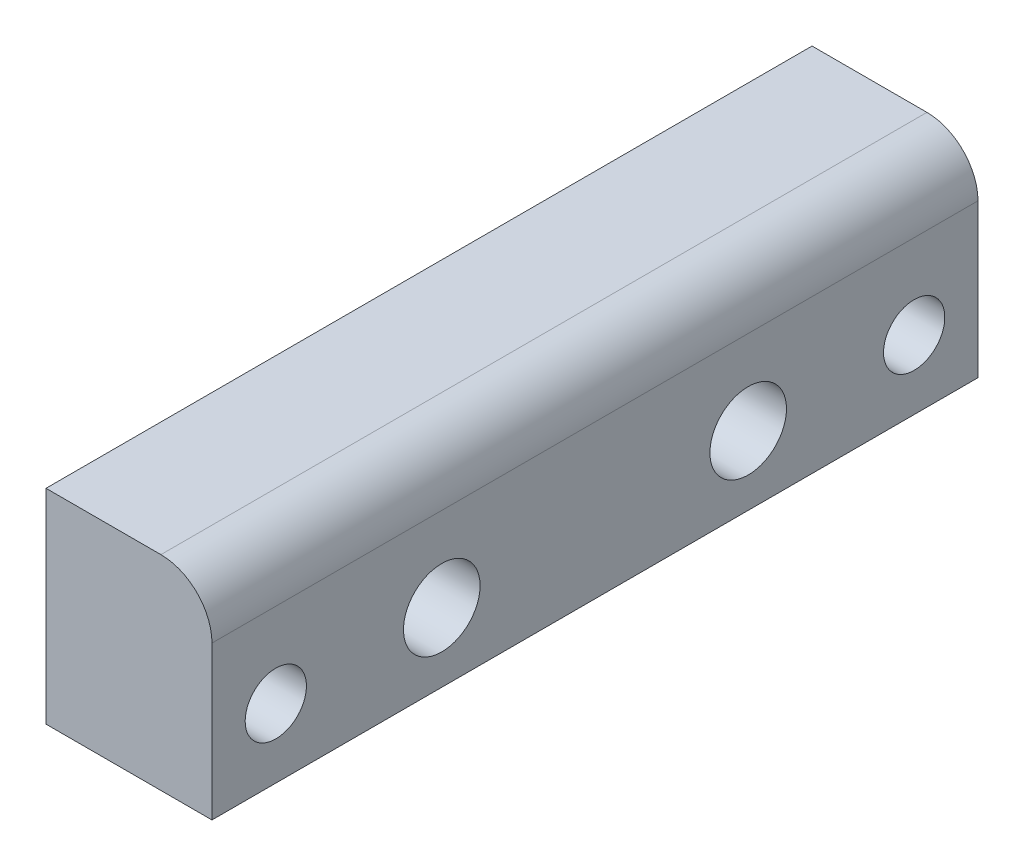
SolidWorks part; units mm, degrees
ref_plane "前视基准面" through (0, 0, 0) normal (0, 0, 1) x (1, 0, 0)
ref_plane "上视基准面" through (0, 0, 0) normal (0, 1, 0) x (1, 0, 0)
ref_plane "右视基准面" through (0, 0, 0) normal (1, 0, 0) x (0, 0, -1)
ref_plane "基准面1" through (3.25, 0, 0) normal (1, 0, 0) x (0, 0, -1)
sketch "草图1" plane through (3.25, 0, 0) normal (1, 0, 0) x (0, 0, -1)
  line L0 (0, -4) -> (0, 4)
  line L1 (0, 4) -> (-30, 4)
  line L2 (-30, 4) -> (-30, -4)
  line L3 (-30, -4) -> (0, -4)
  dimension "D1" = 30
  dimension "D2" = 8
extrude "凸台-拉伸1" add sketch "草图1" against normal blind 6.5
hole_wizard "Ø3.0 (3) 直径孔1" positions "草图3" profile "草图2" hole size "Ø3.0" standard "ANSI Metric"
sketch "草图3" plane through (3.25, 0, 0) normal (1, 0, 0) x (0, 0, -1)
  point P0 (-9, -1.3)
  point P1 (-21, -1.3)
sketch "草图2" plane through (3.25, -1.3, 9) normal (0, 1, 0) x (0, 0, -1)
  line L0 (0, 0) -> (0, 3)
  line L1 (0, 3) -> (1.5, 3)
  line L2 (1.5, 3) -> (1.5, 0)
  line L5 (1.5, 0) -> (0, 0)
  line L10 (0, 3) -> (-1.5, 3) construction
  line L11 (0, -6.35) -> (0, 107.95) construction
  dimension "孔直径" = 3
  dimension "孔深度" = 3
  dimension "导头角度" = 180
hole_wizard "M2 六角头机械螺钉的柱形沉头孔1" positions "草图5" profile "草图4" counterbore size "M2" standard "ANSI Metric"
sketch "草图5" plane through (-3.25, 0, 0) normal (-1, 0, 0) x (0, 0, 1)
  point P0 (27.5, -1.3)
  point P1 (2.5, -1.3)
sketch "草图4" plane through (-3.25, -1.3, 27.5) normal (0, 1, 0) x (0, 0, 1)
  line L0 (0, 0) -> (0, 6.5)
  line L1 (0, 6.5) -> (1.2, 6.5)
  line L3 (1.2, 6.5) -> (1.2, 2)
  line L4 (1.2, 2) -> (2.15, 2)
  line L5 (2.15, 2) -> (2.15, 0)
  line L7 (2.15, 0) -> (0, 0)
  line L11 (0, -6.35) -> (0, 107.95) construction
  dimension "通孔孔直径" = 2.4
  dimension "通孔孔深度" = 6.5
  dimension "柱形沉头孔直径" = 4.3
  dimension "柱形沉头孔深度" = 2
chamfer "倒角1" distance 0.1 angle 44 2 edges at (-3.25, -1.3, 29.65) (-3.25, -1.3, 4.65)
fillet "圆角1" radius 2 1 edges at (3.25, 4, 15)
